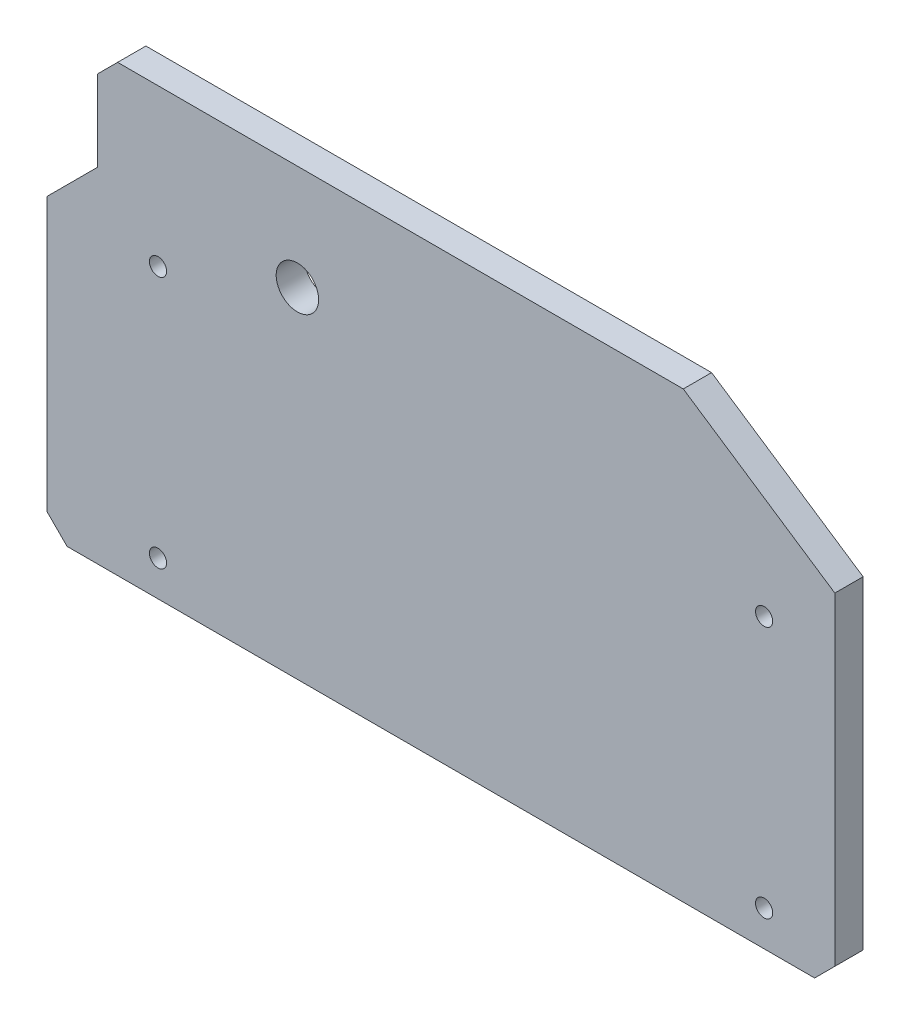
SolidWorks part; units mm, degrees
material "普通碳钢"
ref_plane "Front Plane" through (0, 0, 0) normal (0, 0, 1) x (1, 0, 0)
ref_plane "Top Plane" through (0, 0, 0) normal (0, 1, 0) x (1, 0, 0)
ref_plane "Right Plane" through (0, 0, 0) normal (1, 0, 0) x (0, 0, -1)
sketch "Sketch1" plane through (0, 0, 0) normal (0, 0, 1) x (1, 0, 0)
  line L0 (0, 220) -> (315, 220)
  line L1 (315, 220) -> (390, 170)
  line L2 (390, 170) -> (390, 0)
  line L3 (390, 0) -> (0, 0)
  line L4 (0, 0) -> (0, 220)
  circle A0 centre (124, 168) radius 10.5
  dimension "D11" = 21
  dimension "D3" = 124
  dimension "D1" = 390
  dimension "D2" = 315
  dimension "D7" = 50
  dimension "D9" = 220
  dimension "D12" = 52
extrude "Boss-Extrude1" add sketch "Sketch1" along normal blind 14
hole_wizard "M10 Tapped Hole1" positions "Sketch2" profile "Sketch3" tap size "M10" standard "GB" end condition through all
sketch "Sketch2" plane through (0, 0, 14) normal (0, 0, 1) x (1, 0, 0)
  line L0 (315, 220) -> (0, 220) construction
  line L1 (0, 220) -> (0, 0) construction
  point P0 (55, 142.5)
  point P2 (55, 17.5)
  point P4 (355, 142.5)
  point P6 (355, 17.5)
  dimension "D1" = 77.5
  dimension "D2" = 125
  dimension "D3" = 55
  dimension "D4" = 300
sketch "Sketch3" plane through (55, 142.5, 14) normal (1, 0, 0) x (0, -1, 0)
  line L0 (0, 0) -> (0, 14)
  line L1 (0, 14) -> (4.25, 14)
  line L2 (4.25, 14) -> (4.25, 0)
  line L5 (4.25, 0) -> (0, 0)
  line L11 (0, -6.35) -> (0, 107.95) construction
  dimension "通孔螺纹孔钻头直径" = 8.5
  dimension "通孔螺纹孔钻头深度" = 14
cosmetic thread "Hole thread1" parameters "D2"=10
cosmetic thread "Hole thread2" parameters "D2"=10
cosmetic thread "Hole thread3" parameters "D2"=10
cosmetic thread "Hole thread4" parameters "D2"=10
sketch "Sketch4" plane through (0, 0, 14) normal (0, 0, 1) x (1, 0, 0)
  line L1 (0, 220) -> (25, 220)
  line L2 (0, 220) -> (0, 160)
  line L3 (0, 160) -> (25, 160)
  line L4 (25, 220) -> (25, 160)
  dimension "D1" = 25
  dimension "D2" = 60
extrude "Cut-Extrude1" cut sketch "Sketch4" against normal through all
chamfer "Chamfer1" distance 10 angle 45 4 edges at (390, 0, 7) (0, 0, 7) (25, 220, 7) (25, 160, 7)
sketch "Sketch5" plane through (0, 0, 14) normal (0, 0, 1) x (1, 0, 0)
  line L0 (15, 160) -> (0, 160)
  line L1 (0, 160) -> (0, 145)
  line L2 (0, 160) -> (0, 10) construction
  line L3 (0, 145) -> (15, 160)
  line L4 (25, 170) -> (15, 160) construction
extrude "Cut-Extrude2" cut sketch "Sketch5" against normal through all
